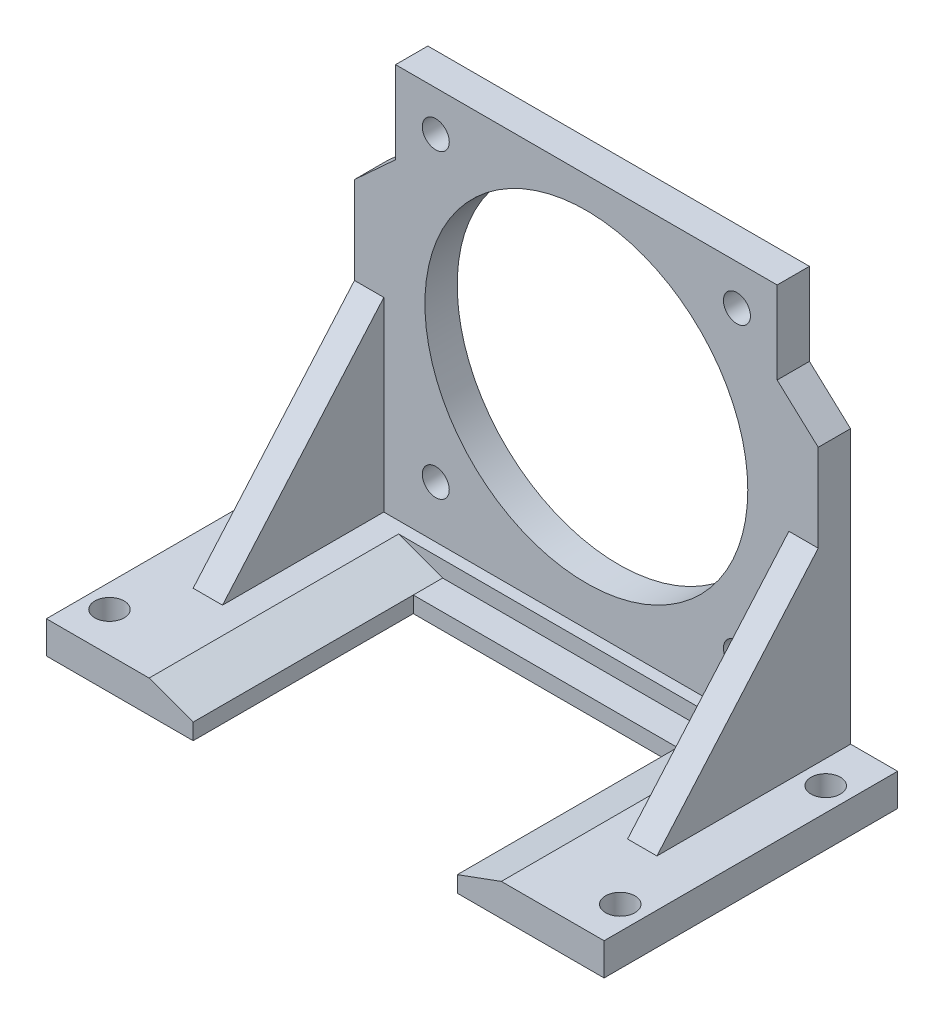
from build123d import *

# Parameters (mm, degrees)
SKETCH_1_W          = 130
SKETCH_1_H          = 130
SKETCH_1_R          = 4.6
SKETCH_1_R_2        = 55
SKETCH_1_H_2        = 4
EXTRUDE_1_DEPTH     = 5.5
SKETCH_2_R          = 5
EXTRUDE_2_DEPTH     = 11
EXTRUDE_3_DEPTH     = 5
CUT_EXTRUDE_1_DEPTH = 85


with BuildPart() as part:
    # 草图1 → 凸台-拉伸1 (new, symmetric)
    # profile 1 of 4: a face of its own
    with BuildSketch(Plane.XY):
        Rectangle(SKETCH_1_W, SKETCH_1_H)
        with Locations((51.3, -51.3)):
            Circle(SKETCH_1_R, mode=Mode.SUBTRACT)
        with Locations((51.3, 51.3)):
            Circle(SKETCH_1_R, mode=Mode.SUBTRACT)
        with Locations((-51.3, 51.3)):
            Circle(SKETCH_1_R, mode=Mode.SUBTRACT)
        with Locations((0, -0.5)):
            Circle(SKETCH_1_R_2, mode=Mode.SUBTRACT)
        with Locations((-51.3, -51.3)):
            Circle(SKETCH_1_R, mode=Mode.SUBTRACT)
    # profile 2 of 4: a face of its own
    with BuildSketch(Plane.XY):
        with Locations((0, -67)):
            Rectangle(SKETCH_1_W, SKETCH_1_H_2)
    # profile 3 of 4: a face of its own
    with BuildSketch(Plane.XY):
        Polygon((-65, -69), (-65, -65), (-65, 36.950223859), (-79, 24.100911478), (-79, 0), (-79, -69), align=None)
    # profile 4 of 4: a face of its own
    with BuildSketch(Plane.XY):
        Polygon((79, 0), (79, 24.100911478), (65, 36.950223859), (65, -65), (65, -69), (79, -69), align=None)
    extrude(amount=EXTRUDE_1_DEPTH, both=True)

    # 草图2 → 凸台-拉伸2 (add)
    with BuildSketch(Plane.XZ.offset(69)):
        Polygon((-95, -5.543155134), (95, -5.543155134), (95, 94.456844866), (45, 94.456844866), (45, 19.456844866), (-45, 19.456844866), (-45, 94.456844866), (-95, 94.456844866), align=None)
        with Locations(Location((-87, 80.956844866, 0), (0, 0, 270))):
            Circle(SKETCH_2_R, mode=Mode.SUBTRACT)
        with Locations(Location((-87, 10.956844866, 0), (0, 0, 270))):
            Circle(SKETCH_2_R, mode=Mode.SUBTRACT)
        with Locations(Location((87, 10.956844866, 0), (0, 0, 90))):
            Circle(SKETCH_2_R, mode=Mode.SUBTRACT)
        with Locations(Location((87, 80.956844866, 0), (0, 0, 90))):
            Circle(SKETCH_2_R, mode=Mode.SUBTRACT)
    extrude(amount=EXTRUDE_2_DEPTH)

    # 草图3 → 凸台-拉伸3 (add, symmetric)
    with BuildSketch(Plane(origin=(74, 0, 0), x_dir=(0, 0, -1), z_dir=(1, 0, 0))):
        Polygon((-5.5, -5.674954384), (-60.456844866, -69), (-5.5, -69), align=None)
    extrude_3 = extrude(amount=EXTRUDE_3_DEPTH, both=True)

    # 镜向1: 凸台-拉伸3 across plane
    add(extrude_3.mirror(Plane(origin=(0, 0, 0), x_dir=(0, 0, 1), z_dir=(1, 0, 0))))

    # 草图4 → 切除-拉伸1 (cut)
    with BuildSketch(Plane.XY.offset(94.456844866)):
        Polygon((-60, -69), (-45, -74.5), (45, -74.5), (60, -69), align=None)
    extrude(amount=-CUT_EXTRUDE_1_DEPTH, mode=Mode.SUBTRACT)


solid = part.part
